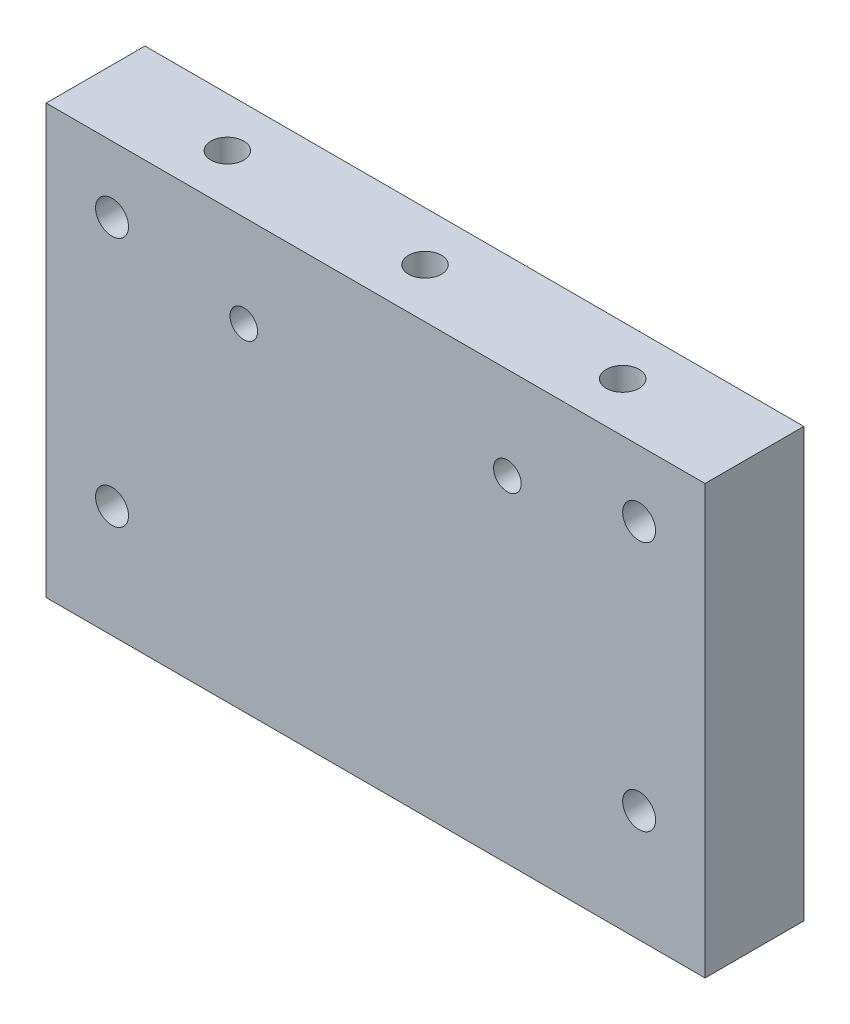
from build123d import *

# Parameters (mm, degrees)
SKETCH_1_W                   = 100
SKETCH_1_H                   = 65
EXTRUDE_1_DEPTH              = 15
HOLE_WIZARD_M6_1_D           = 5
HOLE_WIZARD_M6_1_DEPTH       = 15
HOLE_WIZARD_M6_1_TIP         = 1.502151548
HOLE_WIZARD_M6_2_D           = 5
HOLE_WIZARD_M6_2_DEPTH       = 15
HOLE_WIZARD_M6_2_TIP         = 1.502151548
HOLE_WIZARD_M5_1_D           = 4.2
HOLE_WIZARD_M5_1_CSINK_D     = 5.05
HOLE_WIZARD_M5_1_CSINK_ANGLE = 90
HOLE_WIZARD_M6_3_D           = 5


with BuildPart() as part:
    # 草图1 → 凸台-拉伸1 (new body)
    with BuildSketch(Plane.XY):
        with Locations((50, 32.5)):
            Rectangle(SKETCH_1_W, SKETCH_1_H)
    extrude(amount=EXTRUDE_1_DEPTH)

    # M6 螺纹孔1
    with Locations(Plane(origin=(0, 65, 0), x_dir=(1, 0, 0), z_dir=(0, 1, 0))):
        with Locations((20, -7.5), (80, -7.5), (50, -7.5)):
            Hole(HOLE_WIZARD_M6_1_D / 2, depth=HOLE_WIZARD_M6_1_DEPTH)
            with Locations((0, 0, -(HOLE_WIZARD_M6_1_DEPTH + HOLE_WIZARD_M6_1_TIP / 2))):  # 118° drill point
                Cone(0, HOLE_WIZARD_M6_1_D / 2, HOLE_WIZARD_M6_1_TIP, mode=Mode.SUBTRACT)

    # M6 螺纹孔2
    with Locations(Plane(origin=(0, 0, 0), x_dir=(-1, 0, 0), z_dir=(0, -1, 0))):
        with Locations((-80, -7.5), (-50, -7.5), (-20, -7.5)):
            Hole(HOLE_WIZARD_M6_2_D / 2, depth=HOLE_WIZARD_M6_2_DEPTH)
            with Locations((0, 0, -(HOLE_WIZARD_M6_2_DEPTH + HOLE_WIZARD_M6_2_TIP / 2))):  # 118° drill point
                Cone(0, HOLE_WIZARD_M6_2_D / 2, HOLE_WIZARD_M6_2_TIP, mode=Mode.SUBTRACT)

    # M5 螺纹孔1 (through all)
    with Locations(Plane(origin=(0, 0, 0), x_dir=(-1, 0, 0), z_dir=(0, 0, -1))):
        with Locations((-70, 51), (-30, 51)):
            CounterSinkHole(HOLE_WIZARD_M5_1_D / 2, HOLE_WIZARD_M5_1_CSINK_D / 2, counter_sink_angle=HOLE_WIZARD_M5_1_CSINK_ANGLE)

    # M6 螺纹孔3 (through all)
    with Locations(Plane(origin=(0, 0, 0), x_dir=(-1, 0, 0), z_dir=(0, 0, -1))):
        with Locations((-90, 55), (-10, 55), (-90, 17), (-10, 17)):
            Hole(HOLE_WIZARD_M6_3_D / 2)


solid = part.part
